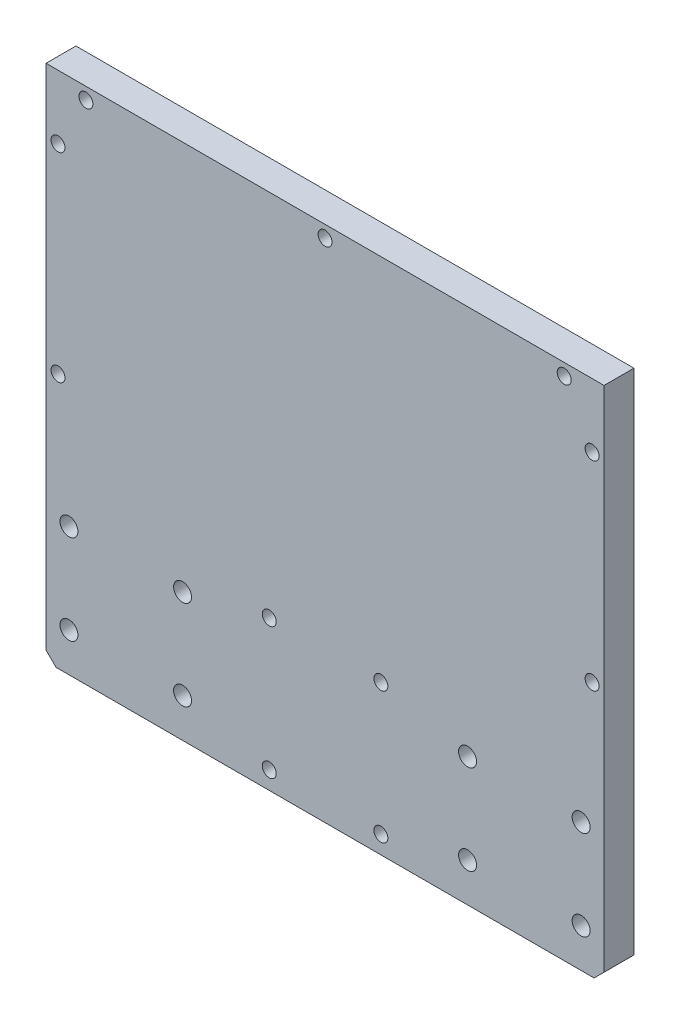
from build123d import *

# Parameters (mm, degrees)
SKETCH_1_W            = 280
SKETCH_1_H            = 260
EXTRUDE_1_DEPTH       = 15
CHAMFER_1_SIZE        = 5
HOLE_WIZARD_7_0_7_3_D = 7
HOLE_WIZARD_7_0_7_2_D = 7
HOLE_WIZARD_9_0_9_1_D = 9
HOLE_WIZARD_7_0_7_1_D = 7


with BuildPart() as part:
    # 草图1 → 凸台-拉伸1 (new body)
    with BuildSketch(Plane.XY):
        with Locations((140, -130)):
            Rectangle(SKETCH_1_W, SKETCH_1_H)
    extrude(amount=EXTRUDE_1_DEPTH)

    # 倒角1
    chamfer_1_edges = [part.edges().sort_by_distance(p)[0] for p in [
        (280, -260, 7.5),
        (0, -260, 7.5),
    ]]
    chamfer(chamfer_1_edges, length=CHAMFER_1_SIZE)

    # Ø7.0 (7) 直径孔3 (through all)
    with Locations(Plane(origin=(0, 0, 0), x_dir=(-1, 0, 0), z_dir=(0, 0, -1))):
        with Locations((-168, -185), (-112, -185), (-112, -251), (-168, -251)):
            Hole(HOLE_WIZARD_7_0_7_3_D / 2)

    # Ø7.0 (7) 直径孔2 (through all)
    with Locations(Plane.XY.offset(15)):
        with Locations((20, -6), (260, -6), (140, -6)):
            Hole(HOLE_WIZARD_7_0_7_2_D / 2)

    # Ø9.0 (9) 直径孔1 (through all)
    with Locations(Plane(origin=(0, 0, 0), x_dir=(-1, 0, 0), z_dir=(0, 0, -1))):
        with Locations((-268.5, -240.5), (-268.5, -195.5), (-211.5, -195.5), (-211.5, -240.5), (-68.5, -240.5), (-68.5, -195.5), (-11.5, -195.5), (-11.5, -240.5)):
            Hole(HOLE_WIZARD_9_0_9_1_D / 2)

    # Ø7.0 (7) 直径孔1 (through all)
    with Locations(Plane.XY.offset(15)):
        with Locations((6, -32), (274, -32), (274, -132), (6, -132)):
            Hole(HOLE_WIZARD_7_0_7_1_D / 2)


solid = part.part
